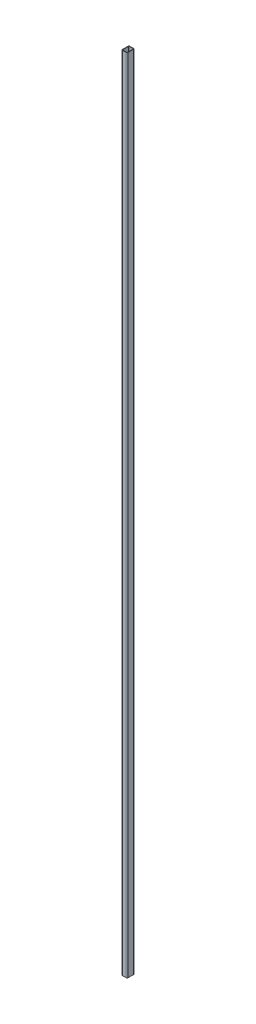
SolidWorks part; units mm, degrees
material "Q235B"
ref_plane "Front Plane" through (0, 0, 0) normal (0, 0, 1) x (1, 0, 0)
ref_plane "Top Plane" through (0, 0, 0) normal (0, 1, 0) x (1, 0, 0)
ref_plane "Right Plane" through (0, 0, 0) normal (1, 0, 0) x (0, 0, -1)
sketch "18 (ProfileFeature) (+7 more in 7 files) Sketch1" plane through (0, 0, 0) normal (0, 0, 1) x (1, 0, 0)
  line L0 (0, 0) -> (0, 8850)
  dimension "D1" = 8850
other "Cold-formed hollow rectangular steel (GB/T 6728-2002) 80×60×5(1)"
ref_plane "Plane1" through (0, 0, 0) normal (0, 1, 0) x (-1, 0, 0)
sketch "Sketch1" plane through (0, 0, 0) normal (0, 1, 0) x (-1, 0, 0)
  line L0 (-20, -35) -> (20, -35)
  line L1 (-25, -30) -> (-25, 30)
  line L2 (20, 35) -> (-20, 35)
  line L3 (25, 30) -> (25, -30)
  line L4 (-20, -40) -> (20, -40)
  line L5 (-30, -30) -> (-30, 30)
  line L6 (20, 40) -> (-20, 40)
  line L7 (30, 30) -> (30, -30)
  arc A0 (30, 30) -> (20, 40) centre (20, 30) ccw
  arc A1 (20, -40) -> (30, -30) centre (20, -30) ccw
  arc A2 (-30, -30) -> (-20, -40) centre (-20, -30) ccw
  arc A3 (-20, 40) -> (-30, 30) centre (-20, 30) ccw
  arc A4 (-20, 35) -> (-25, 30) centre (-20, 30) ccw
  arc A5 (25, 30) -> (20, 35) centre (20, 30) ccw
  arc A6 (20, -35) -> (25, -30) centre (20, -30) ccw
  arc A7 (-25, -30) -> (-20, -35) centre (-20, -30) ccw
  point P0 (0, 40)
  point P1 (30, 0)
  point P2 (0, -40)
  point P3 (-30, 0)
  point P4 (-30, 40)
  point P5 (30, 40)
  point P6 (30, -40)
  point P7 (-30, -40)
  point P8 (0, 0)
  point P33 (0, 0)
  dimension "D1" = 80
  dimension "D2" = 60
  dimension "D3" = 5
  dimension "D4" = 10
